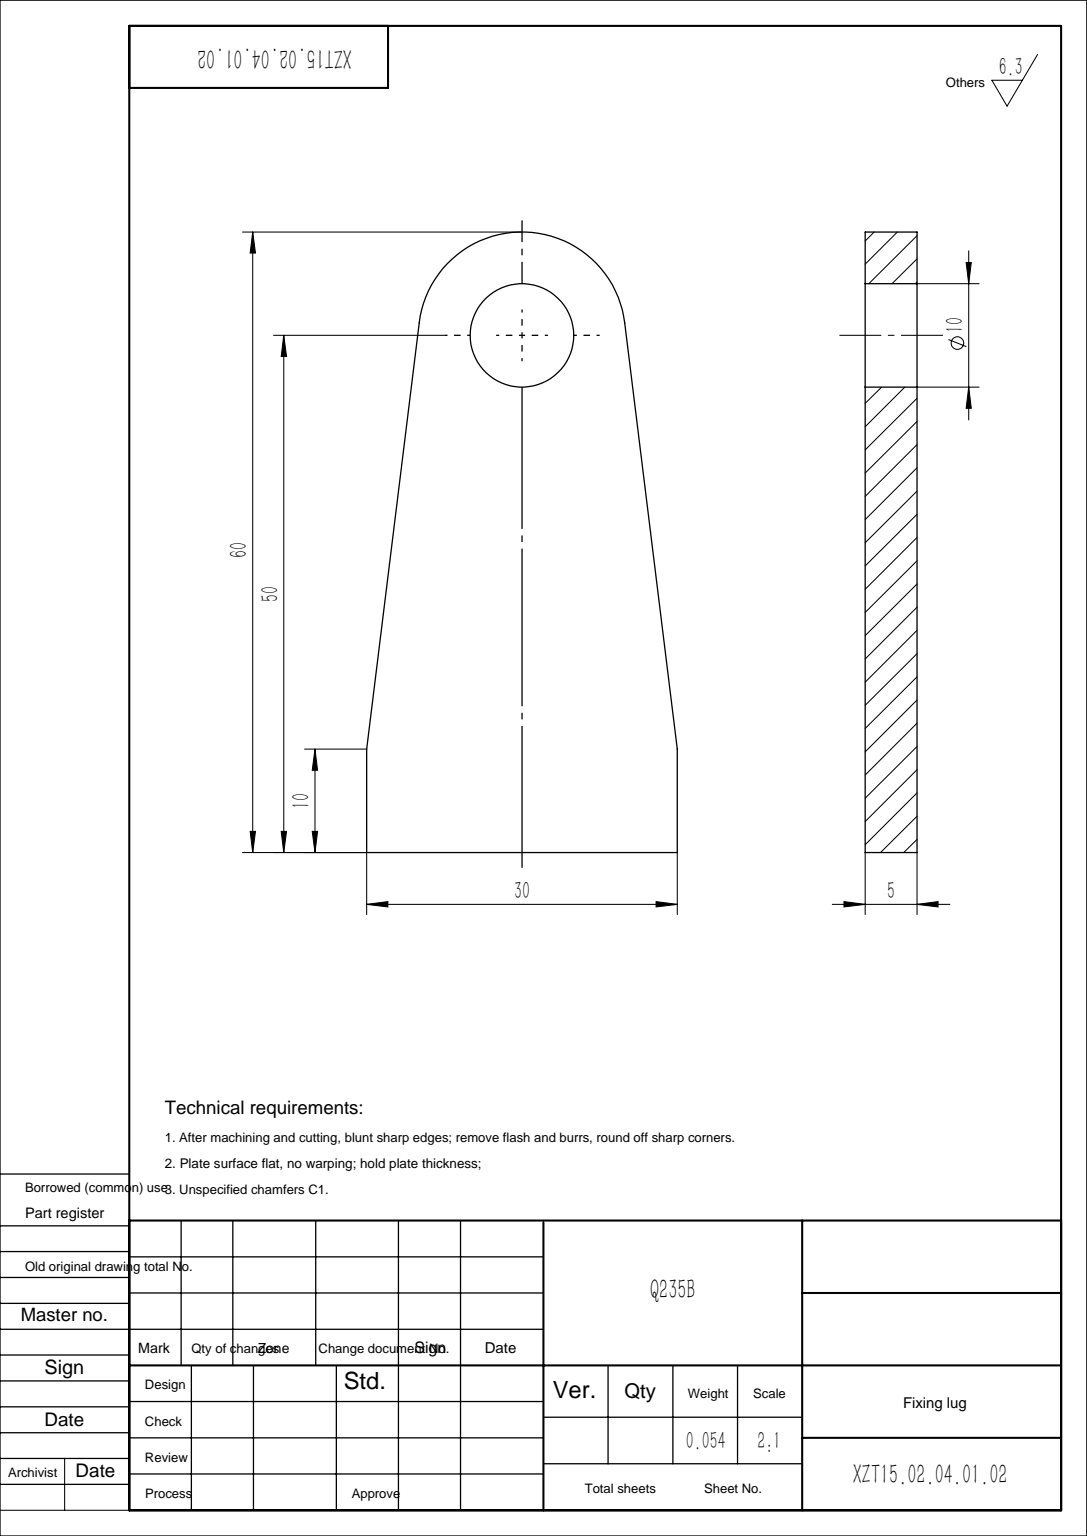
SolidWorks part; units mm, degrees
material "Q235B"
ref_plane "Front Plane" through (0, 0, 0) normal (0, 0, 1) x (1, 0, 0)
ref_plane "Top Plane" through (0, 0, 0) normal (0, 1, 0) x (1, 0, 0)
ref_plane "Right Plane" through (0, 0, 0) normal (1, 0, 0) x (0, 0, -1)
sketch "Sketch1" plane through (0, 0, 0) normal (0, 0, 1) x (1, 0, 0)
  line L0 (15, 0) -> (-15, 0)
  line L1 (-15, 0) -> (-9.9251, 41.2219)
  line L2 (0, 0) -> (0, 40) construction
  line L3 (15, 0) -> (9.9251, 41.2219)
  arc A0 (-9.9251, 41.2219) -> (9.9251, 41.2219) centre (0, 40) cw
  circle A1 centre (0, 40) radius 5
  dimension "D1" = 40
  dimension "D4" = 10
  dimension "D2" = 50
  dimension "D3" = 30
extrude "Boss-Extrude1" add sketch "Sketch1" along normal mid plane 5
sketch "Sketch2" plane through (0, 0, 2.5) normal (0, 0, 1) x (1, 0, 0)
  line L1 (-15, 0) -> (15, 0)
  line L2 (-15, 0) -> (-15, -10)
  line L3 (-15, -10) -> (15, -10)
  line L4 (15, 0) -> (15, -10)
  dimension "D1" = 10
extrude "Boss-Extrude2" add sketch "Sketch2" against normal blind 5
